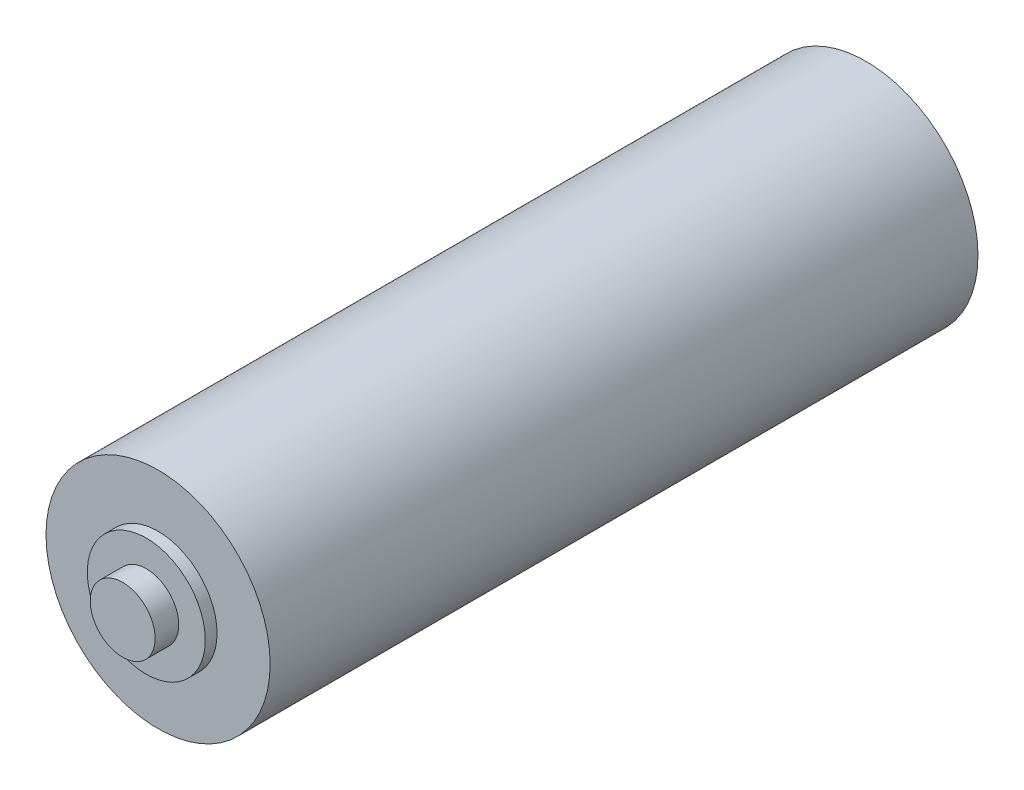
SolidWorks part; units mm, degrees
ref_plane "Front Plane" through (0, 0, 0) normal (0, 0, 1) x (1, 0, 0)
ref_plane "Top Plane" through (0, 0, 0) normal (0, 1, 0) x (1, 0, 0)
ref_plane "Right Plane" through (0, 0, 0) normal (1, 0, 0) x (0, 0, -1)
sketch "Sketch1" plane through (0, 0, 0) normal (0, 0, 1) x (1, 0, 0)
  circle A0 centre (0, 0) radius 95
  dimension "D1" = 190
extrude "Boss-Extrude1" add sketch "Sketch1" along normal blind 600
sketch "Sketch2" plane through (0, 0, 600) normal (0, 0, 1) x (1, 0, 0)
  circle A0 centre (0, 0) radius 50
  dimension "D1" = 100
extrude "Boss-Extrude2" add sketch "Sketch2" along normal blind 10
sketch "Sketch3" plane through (0, 0, 0) normal (0, 0, -1) x (-1, 0, 0)
  circle A0 centre (0, 0) radius 50
  dimension "D1" = 100
extrude "Boss-Extrude3" add sketch "Sketch3" along normal blind 10
sketch "Sketch4" plane through (0, 0, -10) normal (0, 0, -1) x (-1, 0, 0)
  circle A0 centre (0, 0) radius 27.5
  dimension "D1" = 55
extrude "Boss-Extrude4" add sketch "Sketch4" along normal blind 20
sketch "Sketch5" plane through (0, 0, 610) normal (0, 0, 1) x (1, 0, 0)
  circle A0 centre (0, 0) radius 27.5
  dimension "D1" = 55
extrude "Boss-Extrude5" add sketch "Sketch5" along normal blind 20
sketch "Sketch7" plane through (0, 0, 0) normal (0, 0, -1) x (-1, 0, 0)
  circle A0 centre (0, 0) radius 95
